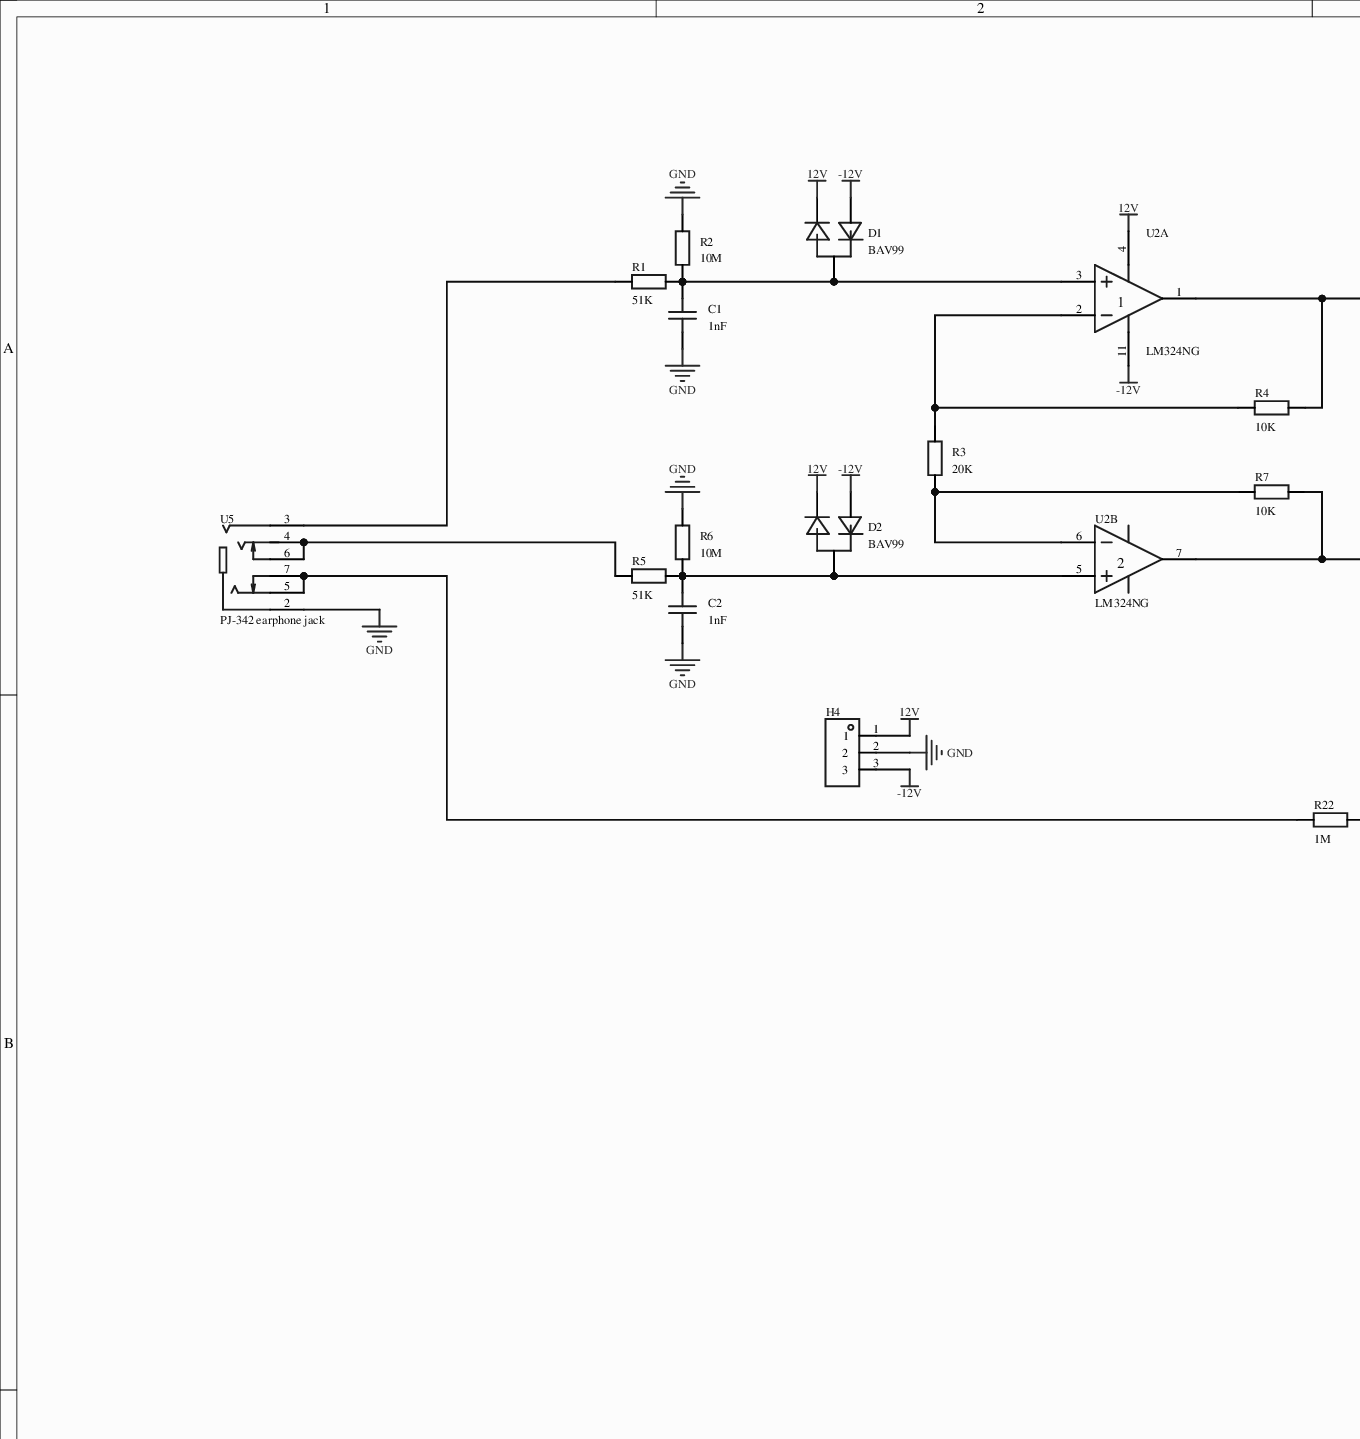
[diagram p0: MISC51578-3.schdoc, top left]
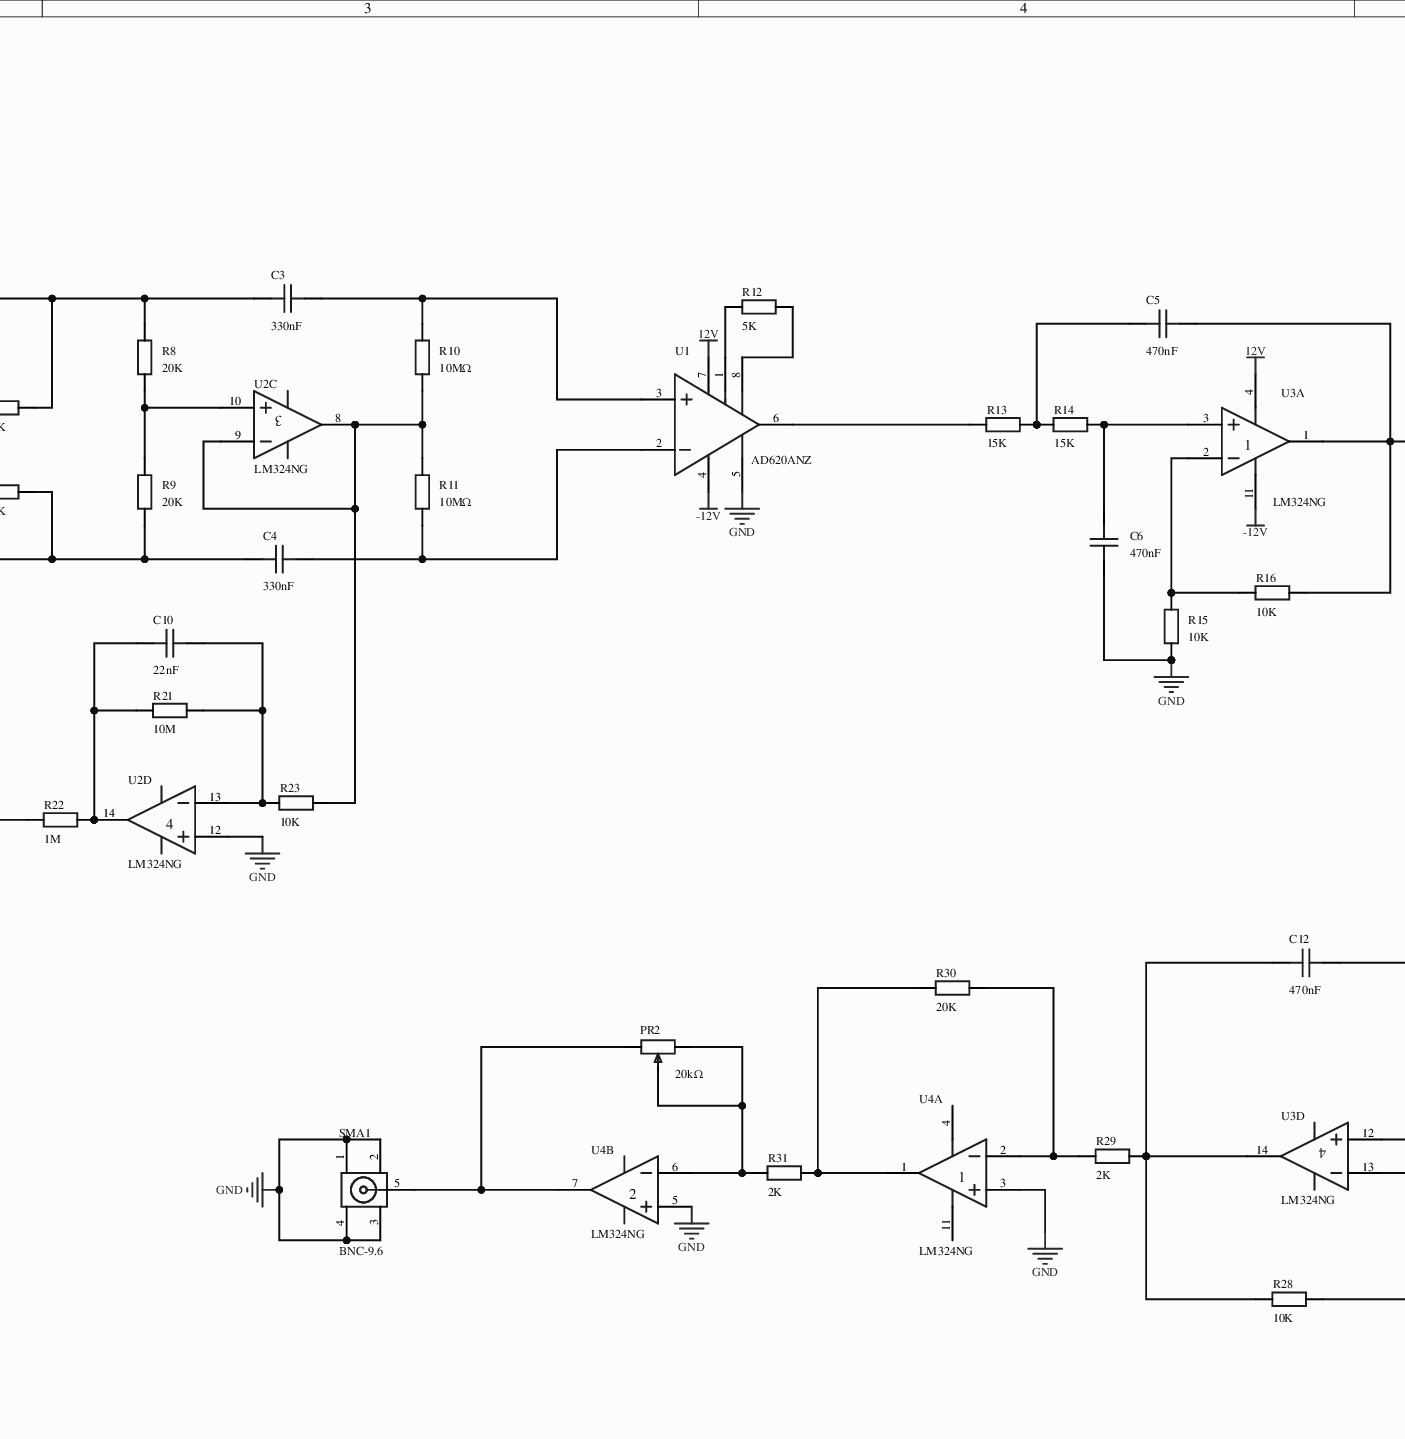
[diagram p1: MISC51578-3.schdoc, top middle]
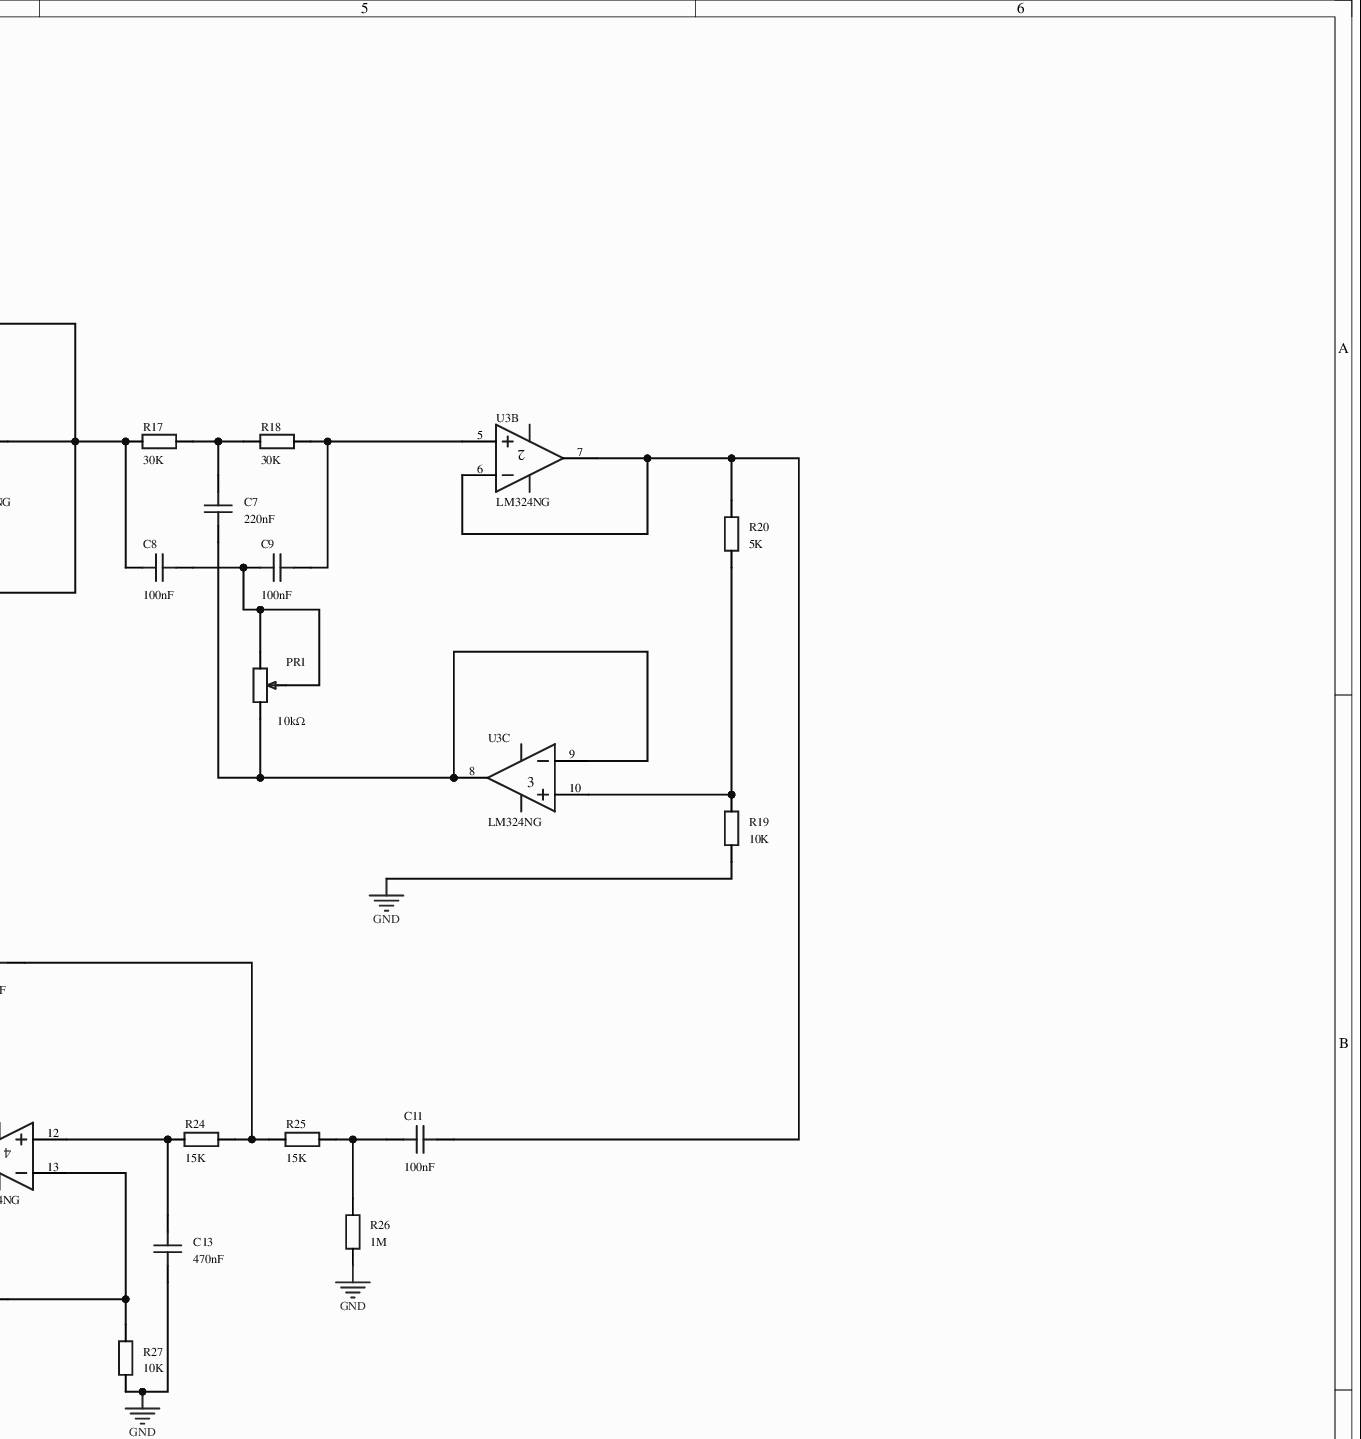
[diagram p2: MISC51578-3.schdoc, top right]
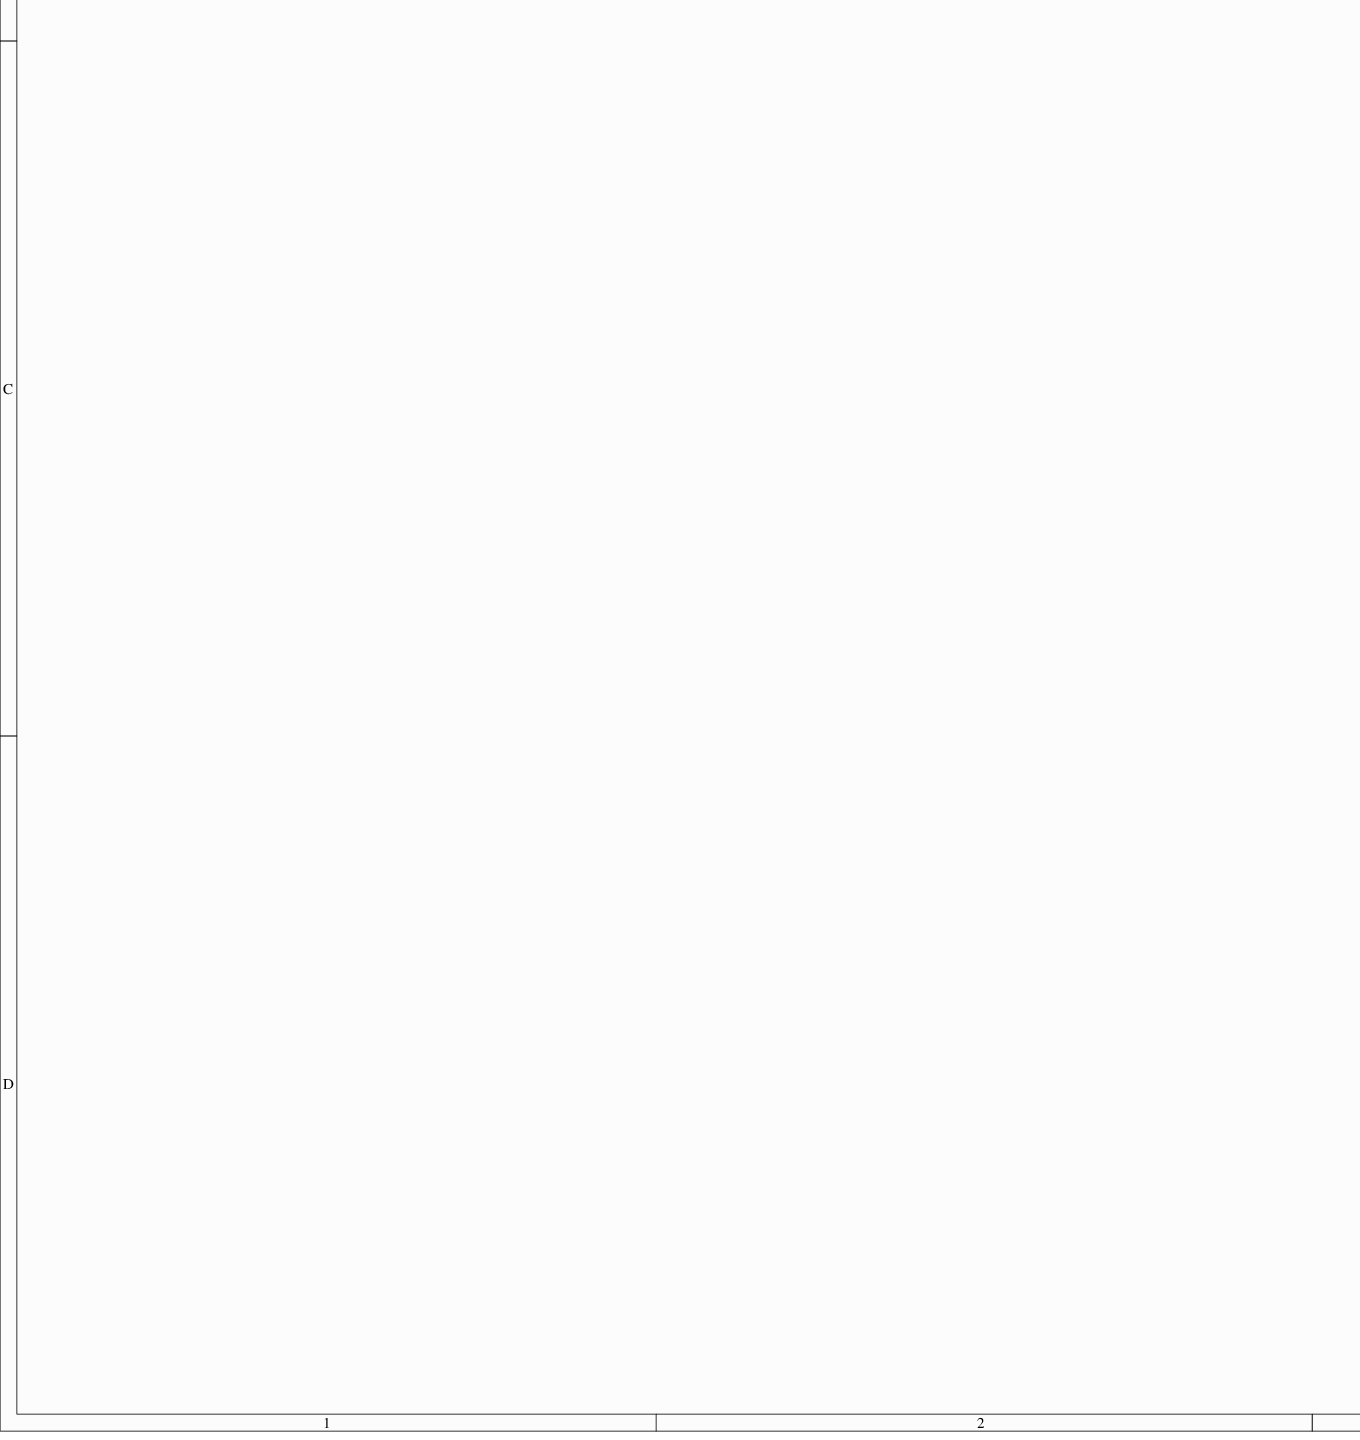
[diagram p3: MISC51578-3.schdoc, bottom left]
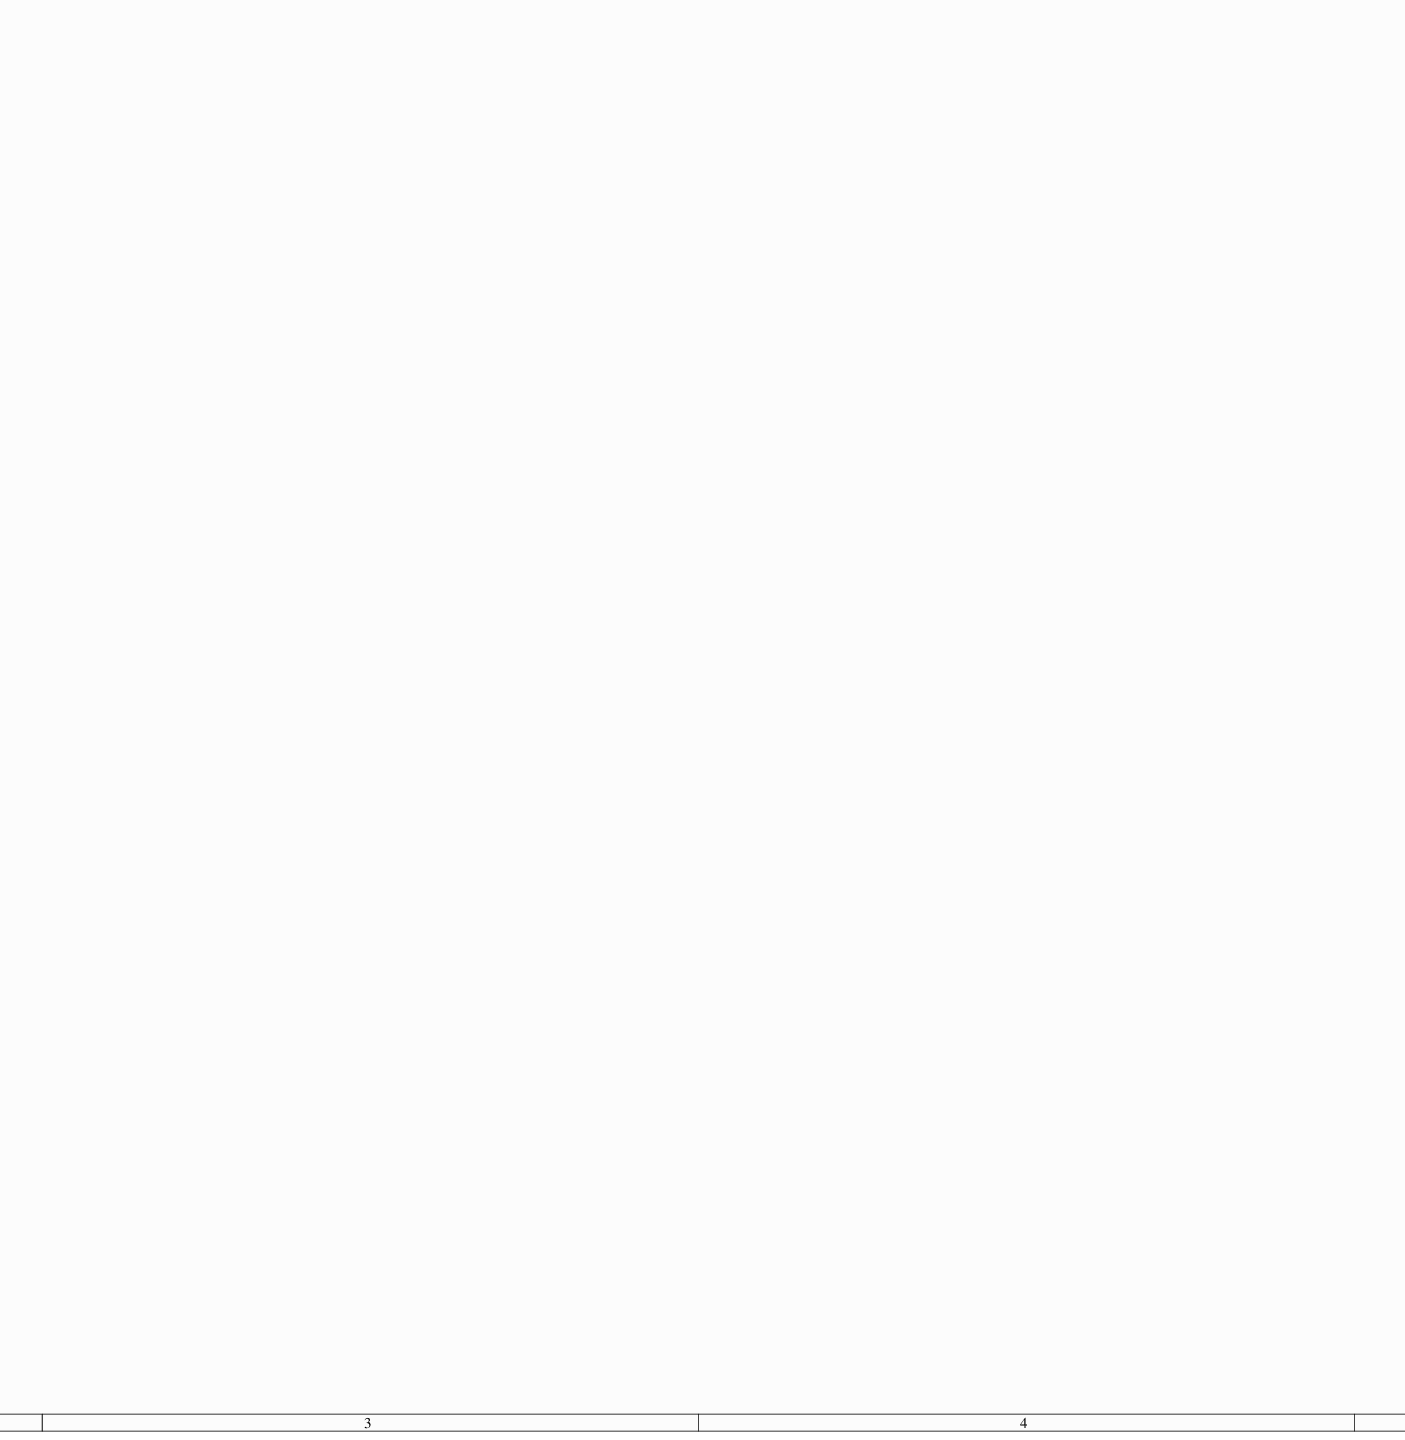
[diagram p4: MISC51578-3.schdoc, bottom middle]
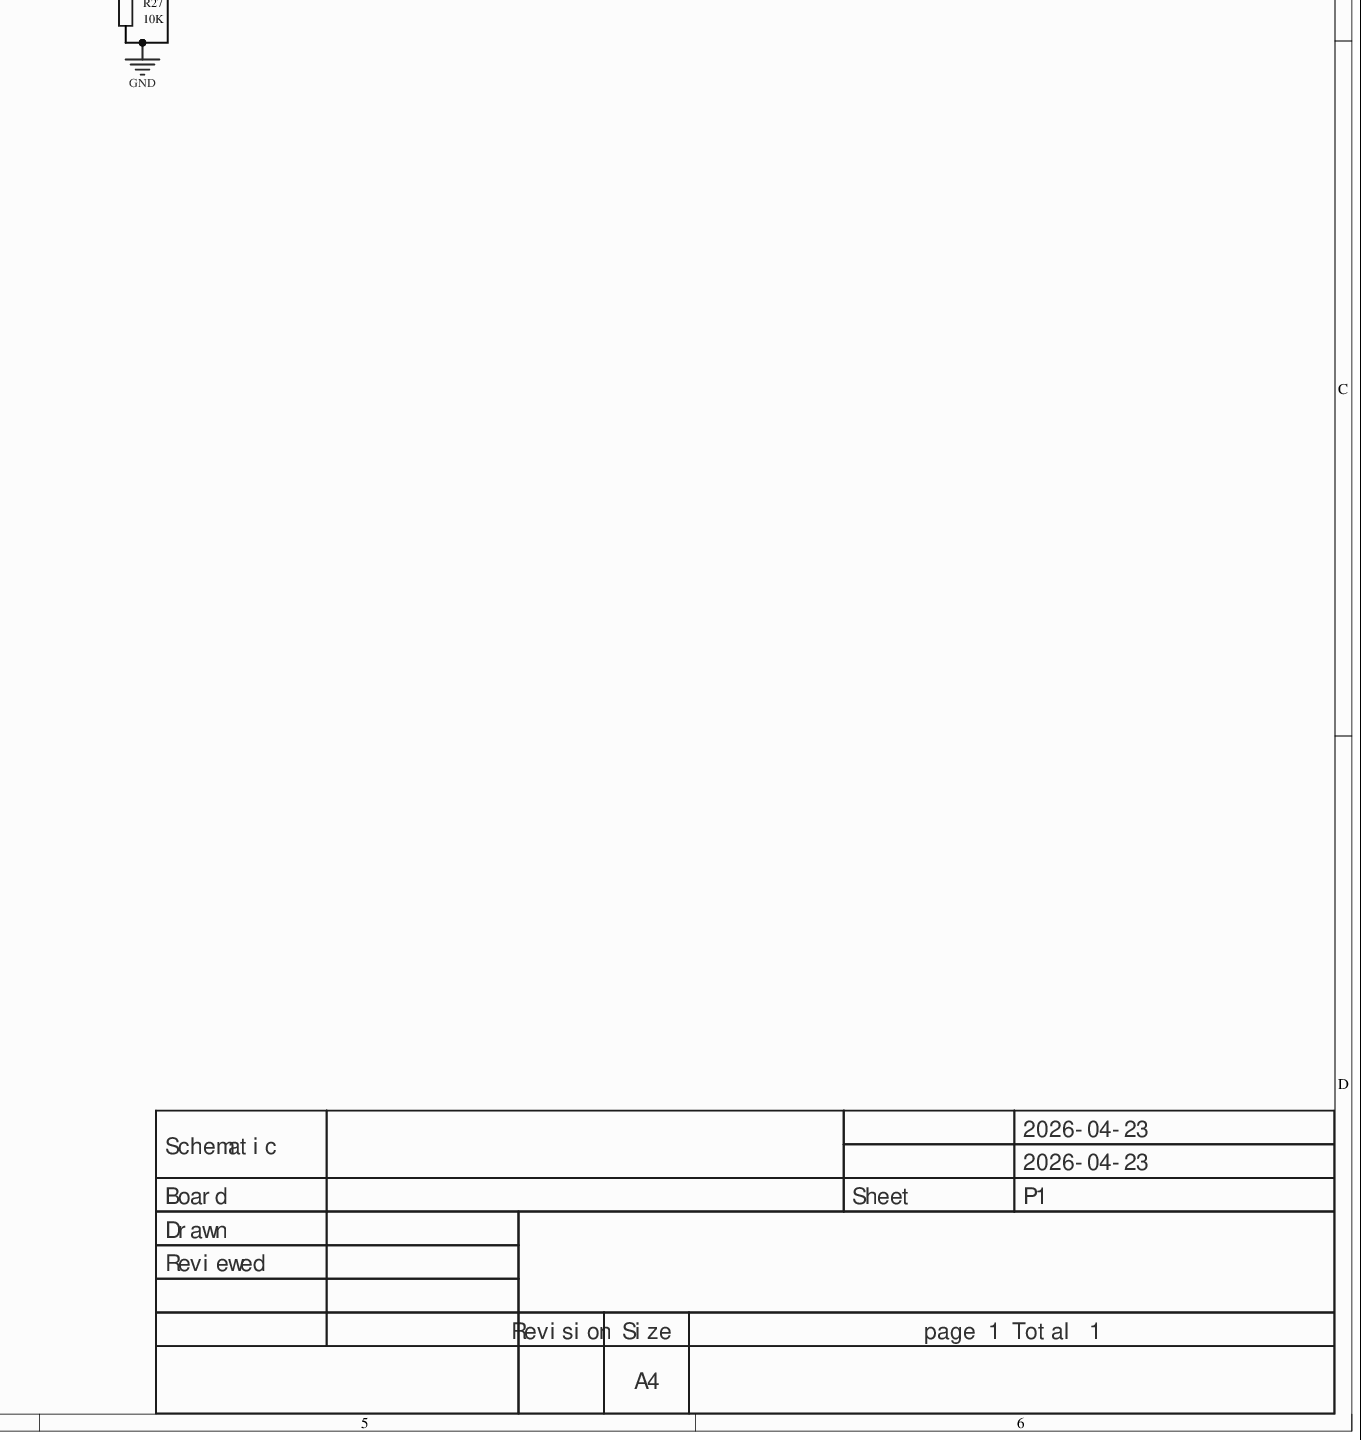
[diagram p5: MISC51578-3.schdoc, bottom right]
# Altium project MISC51578-2.PrjPcb
1 sheet, 55 parts. Net scope: global (net labels, ports and power ports of the same name join across sheets).
Board file: MISC51578.pcbdoc

## Sheet MISC51578-3.schdoc
size 594 x 419 mm; Version: V1.0; @Project Name: MISC51578; @Update Date: 2026-04-23; @Create Date: 2026-04-23; @Board Name: MISC51578; @Create Time: 15:42:31; @Page Count: 1; @Page No: 1; @Schematic Name: MISC51578; @Update Time: 15:42:31; Size: A4

### Parts
C1  1nF  [C0603]
C2  1nF  [C0603]
C3  330nF  [C0603]
C4  330nF  [C0603]
C5  470nF  [C0603]
C6  470nF  [C0603]
C7  220nF  [C0603]
C8  100nF  [C0603]
C9  100nF  [C0603]
C10  22nF  [C0603]
C11  100nF  [C0603]
C12  470nF  [C0603]
C13  470nF  [C0603]
D1  BAV99  [SOT-23-3_L2.9-W1.3-P1.90-LS2.4-BR]
D2  BAV99  [SOT-23-3_L2.9-W1.3-P1.90-LS2.4-BR]
H4  (no value)  [HDR-TH_3P-P2.54-V-M]
PR1  10kΩ  [R_3296]
PR2  20kΩ  [R_3296]
R1  51K  [R0603]
R2  10M  [R0603]
R3  20K  [R0603]
R4  10K  [R0603]
R5  51K  [R0603]
R6  10M  [R0603]
R7  10K  [R0603]
R8  20K  [R0603]
R9  20K  [R0603]
R10  10MΩ  [R0603]
R11  10MΩ  [R0603]
R12  5K  [R0603]
R13  15K  [R0603]
R14  15K  [R0603]
R15  10K  [R0603]
R16  10K  [R0603]
R17  30K  [R0603]
R18  30K  [R0603]
R19  10K  [R0603]
R20  5K  [R0603]
R21  10M  [R0603]
R22  1M  [R0603]
R23  10K  [R0603]
R24  15K  [R0603]
R25  15K  [R0603]
R26  1M  [R0603]
R27  10K  [R0603]
R28  10K  [R0603]
R29  2K  [R0603]
R30  20K  [R0603]
R31  2K  [R0603]
SMA1  BNC-9.6  [SMA-TH_5P_BNC-9.6]
U1  AD620ANZ  [DIP-8_L9.3-W6.4-P2.54-LS7.6-BL]
U2  LM324NG  [PDIP-14_L19.7-W6.6-P2.54-LS8.3-BL]  (parts A,B,C,D of 4)
U3  LM324NG  [PDIP-14_L19.7-W6.6-P2.54-LS8.3-BL]  (parts A,B,C,D of 4)
U4  LM324NG  [PDIP-14_L19.7-W6.6-P2.54-LS8.3-BL]  (parts A,B of 4)
U5  PJ-342 earphone jack  [AUDIO-SMD_PJ-342_C9900012319]

### Nets
12V: D1.2 D2.2 H4.1 U1.7(+VS) U2.4(VCC) U3.4(VCC)
-12V: D1.1 D2.1 H4.3 U1.4(-VS) U2.11(GND) U3.11(GND)
GND: C1.1 C2.1 C6.1 C13.1 H4.2 R2.2 R6.2 R15.1 R19.1 R26.1 R27.1 SMA1.1 SMA1.2 SMA1.3 SMA1.4 U1.5(REF) U2.12(IN4+) U4.3(IN1+) U4.5(IN2+) U5.2
NetC1_2: C1.2 D1.3 R1.2 R2.1 U2.3(IN1-)
NetC2_2: C2.2 D2.3 R5.2 R6.1 U2.5(IN2+)
NetC3_1: C3.1 R4.1 R8.2 U2.1(OUT1)
NetC3_2: C3.2 R10.2 U1.3(+IN)
NetC4_1: C4.1 R7.1 R9.1 U2.7(OUT2)
NetC4_2: C4.2 R11.1 U1.2(-IN)
NetC5_1: C5.1 R13.2 R14.1
NetC5_2: C5.2 C8.2 R16.1 R17.1 U3.1(OUT1)
NetC6_2: C6.2 R14.2 U3.3(IN1-)
NetC7_1: C7.1 PR1.1 U3.8(OUT3) U3.9(IN3-)
NetC7_2: C7.2 R17.2 R18.1
NetC8_1: C8.1 C9.2 PR1.2 PR1.3
NetC9_1: C9.1 R18.2 U3.5(IN2+)
NetC10_1: C10.1 R21.1 R22.2 U2.14(OUT4)
NetC10_2: C10.2 R21.2 R23.1 U2.13(IN4-)
NetC11_1: C11.1 R25.2 R26.2
NetC11_2: C11.2 R20.2 U3.6(IN2-) U3.7(OUT2)
NetC12_1: C12.1 R28.2 R29.2 U3.14(OUT4)
NetC12_2: C12.2 R24.2 R25.1
NetC13_2: C13.2 R24.1 U3.12(IN4+)
NetPR2_1: PR2.1 SMA1.5 U4.7(OUT2)
NetPR2_2: PR2.2 PR2.3 R31.1 U4.6(IN2-)
NetR1_1: R1.1 U5.3
NetR3_1: R3.1 R7.2 U2.6(IN2-)
NetR3_2: R3.2 R4.2 U2.2(IN1+)
NetR5_1: R5.1 U5.4 U5.6
NetR8_1: R8.1 R9.2 U2.10(IN3+)
NetR10_1: R10.1 R11.2 R23.2 U2.8(OUT3) U2.9(IN3-)
NetR12_1: R12.1 U1.1(RG)
NetR12_2: R12.2 U1.8(RG)
NetR13_1: R13.1 U1.6(OUTPUT)
NetR15_2: R15.2 R16.2 U3.2(IN1+)
NetR19_2: R19.2 R20.1 U3.10(IN3+)
NetR22_1: R22.1 U5.5 U5.7
NetR27_2: R27.2 R28.1 U3.13(IN4-)
NetR29_1: R29.1 R30.2 U4.2(IN1-)
NetR30_1: R30.1 R31.2 U4.1(OUT1)

Not connected (* = marked no-connect by the designer): U4 4(VCC) 11(GND)

### Notes on the sheet
- 2026-04-23
- Schematic
- Board
- Sheet
- P1
- Drawn
- Reviewed
- Revision
- Size
- A4
- page 1 Total 1

### Library data of the parts
C1-C13 = CAP_0603: Symbol: Capacitance; ConvertToPcb: yes; ModelId: ac125912035d415993ca9572d50418b10819f05c4eef4c71ace90d822a990e87; ModelName: C0603_L1.6-W0.8-H0.8; ModelTransform: 62.992,31.496,0,0,0,0,0,0,0; Device: CAP_0603; AddInBom: yes; Supplier Footprint: 0603; FootprintName: C0603
  C1 C2: Value: 1nF
  C3 C4: Value: 330nF
  C5 C6 C12 C13: Value: 470nF
  C7: Value: 220nF
  C8 C9 C11: Value: 100nF
  C10: Value: 22nF
D1 D2 = BAV99_C458983: Diode configuration: 1 pair in series; forward voltage (Vf): 1.25V; DC reverse voltage (Vr): 75V; rectified current: 215mA; reverse recovery time (Trr): 4ns;; Manufacturer: Slkor(萨科微); AddInBom: yes; ModelId: c62791f0466c4ae2a892c056b845b0ca0819f05c4eef4c71ace90d822a990e87; ModelName: SOT-23-3P_L2.9-W1.3-H1.0-LS2.4-P0.95; ModelTransform: 98.425,114.173,0,180,0,0,0.0005,-0.0005,0; Pd - Power Dissipation: 350mW; Non-Repetitive Peak Forward Surge Current: 4.5A; Symbol: BAV99_C458983; Device: BAV99_C458983; LCSC Part Name: BAV99; SupplierPart: C458983; ManufacturerPart: BAV99; Supplier Footprint: SOT-23; JLCPCB Part Class: Extended Part; Datasheet: https://example.com/datasheet/BAV99/463066.html; Supplier: LCSC; ConvertToPcb: yes; FootprintName: SOT-23-3_L2.9-W1.3-P1.90-LS2.4-BR; Diode Configuration: 1 pair in series; Voltage - Forward(Vf@If): 1.25V; Voltage - DC Reverse(Vr): 75V; Current - Rectified: 215mA; Reverse Leakage Current (Ir): -; Reverse Recovery Time (trr): 4ns; Operating Junction Temperature Range: -
H4 = HDR-M_2.54_1x3P: AddInBom: yes; ModelId: bb473b6d38ff42a99216a4fcdbdcc4cb0819f05c4eef4c71ace90d822a990e87; ModelName: HDR-TH_3P-P2.54-M-LI-1X3P; ModelTransform: 300.03877,100,0,0,0,0,0,0,-118.11; Symbol: HDR-M_2.54_1x3P; Device: HDR-M_2.54_1x3P; ConvertToPcb: yes; FootprintName: HDR-TH_3P-P2.54-V-M; SupplierPart: C2937625; Supplier Footprint: 插件
PR1 PR2 = R_3296: ConvertToPcb: yes; ModelId: b182808559bb43bda9e7de64b64134cb0819f05c4eef4c71ace90d822a990e87; ModelName: 3296W; ModelTransform: 373.98,188.96,590.49,180,0,0,0,0,-140; Symbol: R_3296; Device: R_3296; AddInBom: yes; Supplier Footprint: 直插; FootprintName: R_3296
  PR1: Value: 10kΩ
  PR2: Value: 20kΩ
R1-R31 = Res_0603: Symbol: Resistor; ConvertToPcb: yes; ModelId: fc143cca1e79419f9cd78b61e9279f080819f05c4eef4c71ace90d822a990e87; ModelTransform: 31.8897,63.7794,0,90,0,0,0,0,0; Device: Res_0603; AddInBom: yes; Supplier Footprint: 0603; FootprintName: R0603; ModelName: R0603
  R1 R5: Value: 51K
  R2 R6 R21: Value: 10M
  R3 R8 R9 R30: Value: 20K
  R4 R7 R15 R16 R19 R23 R27 R28: Value: 10K
  R10 R11: Value: 10MΩ
  R12 R20: Value: 5K
  R13 R14 R24 R25: Value: 15K
  R17 R18: Value: 30K
  R22 R26: Value: 1M
  R29 R31: Value: 2K
SMA1 = BNC-9.6: AddInBom: yes; ModelId: 168d17ae366a4f42a983146d83702d210819f05c4eef4c71ace90d822a990e87; ModelTransform: 1141.73,529.68,0,0,0,0,-373.424,0,-157.48; Symbol: BNC-9.6; Device: BNC-9.6; LCSC Part Name: BNC-9.6; SupplierPart: C9900020578; ManufacturerPart: BNC-9.6; Supplier Footprint: BNC-9.6; JLCPCB Part Class: Extended Part; Supplier: LCSC; ConvertToPcb: yes; FootprintName: SMA-TH_5P_BNC-9.6; ModelName: SMA-TH_5P_BNC-9.6
U1 = AD620ANZ: Amplifiers: single; common-mode rejection ratio (CMRR): 100dB; input bias current (Ib): 500pA; input offset voltage (Vos): 30uV; gain-bandwidth product (GBP): -; slew rate (SR): 0.75V/us; bandwidth (-3dB): 120kHz;; Manufacturer: ADI(亚德诺); AddInBom: yes; ModelId: e1ba2ac1384341a197ae27979c8d89420819f05c4eef4c71ace90d822a990e87; ModelName: DIP-8_L9.3-W6.4-H4.5-P2.54-LS7.6-BL; ModelTransform: 364.173,311.8104,0,0,0,0,0,0,-118.11; Voltage - Supply: 2.3V~18V; -18V~-2.3V; Output Current: 18mA; Quiescent Current per Amplifier: 1.3mA; Input Offset Voltage Drift(Vos TC): 0.3uV/℃; Symbol: AD620ANZ; Device: AD620ANZ; LCSC Part Name: 低成本低功耗仪表放大器; SupplierPart: C9680; ManufacturerPart: AD620ANZ; Supplier Footprint: DIP-8; JLCPCB Part Class: Extended Part; Datasheet: https://example.com/datasheet/AD620ANZ/10210.html; Supplier: LCSC; ConvertToPcb: yes; FootprintName: DIP-8_L9.3-W6.4-P2.54-LS7.6-BL; Number of Channels: Single; Common Mode Rejection Ratio(CMRR): 100dB; Ib - Input Bias Current: 500pA; Vos - Input Offset Voltage: 30uV; Gain Bandwidth Product: -; Slew Rate: 0.75V/us; -3dB Bandwidth: 120kHz; Operating Temperature: -40℃~+85℃
U2-U4 = LM324NG: Amplifiers: 4; rail-to-rail: -; gain-bandwidth product (GBW): -; input offset voltage (Vos): 5mV; slew rate (SR): 600V/ms; input bias current (Ib): 300nA;; Manufacturer: onsemi(安森美); Relevance: []; AddInBom: yes; ModelId: 94f7bce1495f46559ec9e5ea41bd66480819f05c4eef4c71ace90d822a990e87; ModelName: PDIP-14_L19.7-W6.6-H5.1-P2.54-LS8.3-BL; ModelTransform: 755.904,339.369,0,0,0,0,0,0,-118.11; Number of Channels: 4; Maximum Power Supply Range (Vdd-Vss): 32V; Input Offset Voltage Drift(Vos TC): 7uV/℃; Input Offset Current(Ios): 5nA; Common Mode Rejection Ratio(CMRR): 85dB; Output Current: 40mA; Single supply: 3V~32V; Dual Supply: -16V~16V; Symbol: LM324NG; Device: LM324NG; LCSC Part Name: 停产 LM324NG; SupplierPart: C99121; ManufacturerPart: LM324NG; Supplier Footprint: PDIP-14; JLCPCB Part Class: Extended Part; Datasheet: https://example.com/datasheet/LM324NG/100334.html; Supplier: LCSC; ConvertToPcb: yes; FootprintName: PDIP-14_L19.7-W6.6-P2.54-LS8.3-BL; Rail to Rail: -; Gain Bandwidth Product: -; Vos - Input Offset Voltage: 5mV; Slew Rate: 600V/ms; Ib - Input Bias Current: 300nA; Input Voltage Noise Density: -; Input offset current drift(Ios TC): -; Quiescent Current: -; Operating Temperature: 0℃~+70℃; Features: -
U5 = PJ-342耳机座: AddInBom: yes; ModelId: 74245672669e454d9033d3b0ffaf50180819f05c4eef4c71ace90d822a990e87; ModelTransform: 551.18,334.645,0,0,0,0,-84.646,0,-23.622; Symbol: PJ-342 earphone jack; Device: PJ-342 earphone jack; LCSC Part Name: PJ-342耳机座; SupplierPart: C9900012319; ManufacturerPart: PJ-342耳机座; Supplier Footprint: SMD; JLCPCB Part Class: Extended Part; Supplier: LCSC; ConvertToPcb: yes; FootprintName: AUDIO-SMD_PJ-342_C9900012319; ModelName: AUDIO-SMD_PJ-342_C9900012319